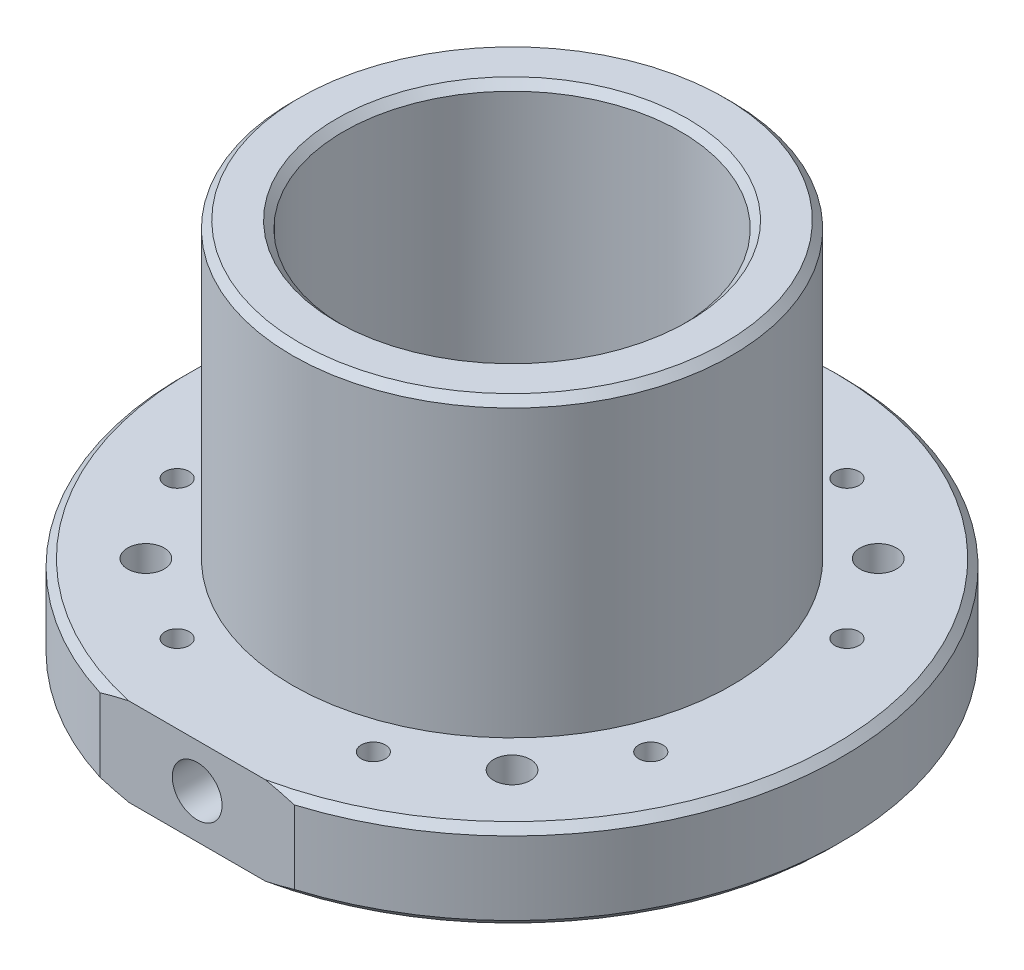
from build123d import *

# Parameters (mm, degrees)
SKETCH1_R              = 45
BOSS_EXTRUDE1_DEPTH    = 12
SKETCH2_R              = 30
BOSS_EXTRUDE2_DEPTH    = 40
SKETCH3_R              = 23
CUT_EXTRUDE1_DEPTH     = 83.182723245
CHAMFER1_SIZE          = 1
M6_TAPPED_HOLE1_D      = 5
M4_TAPPED_HOLE1_D      = 3.3
CUT_EXTRUDE2_DEPTH     = 83.182723245
CIRPATTERN1_COUNT      = 8
M8_TAPPED_HOLE1_REACH  = 113.683
M8_TAPPED_HOLE1_BORE_R = 3.4


with BuildPart() as part:
    # Sketch1 → Boss-Extrude1 (new body)
    with BuildSketch(Plane(origin=(0, 0, 0), x_dir=(1, 0, 0), z_dir=(0, 1, 0))):
        with Locations(Location((0, 0, 0), (0, 0, 270))):
            Circle(SKETCH1_R)
    extrude(amount=BOSS_EXTRUDE1_DEPTH)

    # Sketch2 → Boss-Extrude2 (add)
    with BuildSketch(Plane(origin=(0, 12, 0), x_dir=(1, 0, 0), z_dir=(0, 1, 0))):
        with Locations(Location((0, 0, 0), (0, 0, 270))):
            Circle(SKETCH2_R)
    extrude(amount=BOSS_EXTRUDE2_DEPTH)

    # Sketch3 → Cut-Extrude1 (cut, through all)
    with BuildSketch(Plane.XZ):
        with Locations(Location((0, 0, 0), (0, 0, 270))):
            Circle(SKETCH3_R)
    extrude(amount=-CUT_EXTRUDE1_DEPTH, mode=Mode.SUBTRACT)

    # Chamfer1
    chamfer1_edges = [part.edges().sort_by_distance(p)[0] for p in [
        (0, 52, 23),
        (0, 0, 23),
        (0, 0, -45),
        (0, 12, -45),
        (0, 52, -30),
    ]]
    chamfer(chamfer1_edges, length=CHAMFER1_SIZE)

    # M6 Tapped Hole1 (through all)
    with Locations(Plane(origin=(0, 0, 0), x_dir=(-1, 0, 0), z_dir=(0, -1, 0))):
        with Locations((25, -25), (-25, -25), (-25, 25), (25, 25)):
            Hole(M6_TAPPED_HOLE1_D / 2)

    # M4 Tapped Hole1 (through all)
    with Locations(Plane(origin=(0, 0, 0), x_dir=(-1, 0, 0), z_dir=(0, -1, 0))):
        with Locations((13.393920133, -32.335783638)):
            m4_tapped_hole1 = Hole(M4_TAPPED_HOLE1_D / 2)

    # Sketch8 → Cut-Extrude2 (cut, through all)
    with BuildSketch(Plane.XZ):
        with BuildLine():
            Line((-13.266499161, 43), (13.266499161, 43))
            ThreePointArc((13.266499161, 43), (0, 45), (-13.266499161, 43))
        make_face()
    extrude(amount=-CUT_EXTRUDE2_DEPTH, mode=Mode.SUBTRACT)

    # CirPattern1: M4 Tapped Hole1 ×8 about axis
    cirpattern1_axis = Axis((0, 0, 0), (0, 1, 0))
    for i in range(1, CIRPATTERN1_COUNT):
        add(m4_tapped_hole1.rotate(cirpattern1_axis, i * 360 / CIRPATTERN1_COUNT), mode=Mode.SUBTRACT)

    # M8 Tapped Hole1 bore → M8 Tapped Hole1 (cut, up to next)
    with BuildSketch(Plane.XY.offset(43), mode=Mode.PRIVATE) as m8_tapped_hole1_sk1:
        with Locations((0, 6)):
            Circle(M8_TAPPED_HOLE1_BORE_R)
    m8_tapped_hole1_tool1 = extrude(m8_tapped_hole1_sk1.sketch, amount=-M8_TAPPED_HOLE1_REACH, mode=Mode.PRIVATE) & part.part
    add(m8_tapped_hole1_tool1.solids().sort_by_distance((0, 6, 43))[0], mode=Mode.SUBTRACT)


solid = part.part
